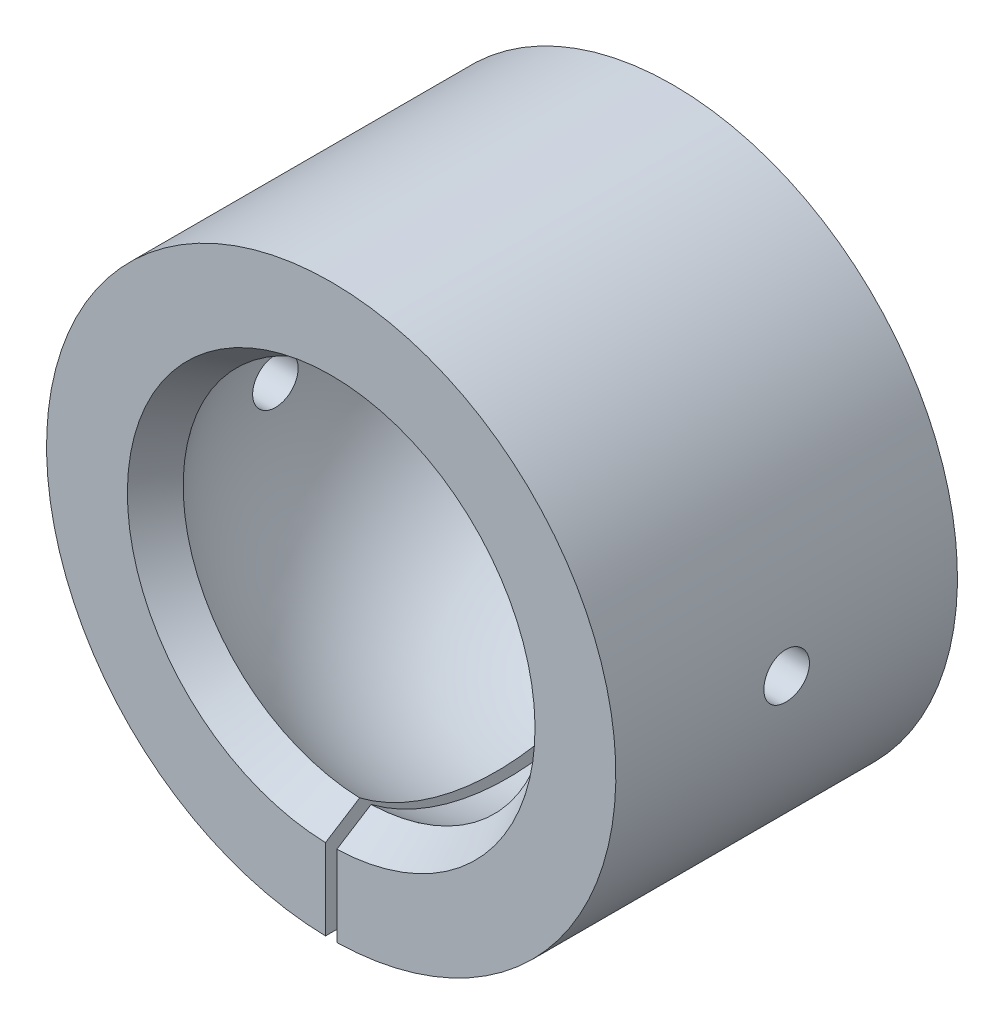
from build123d import *

# Parameters (mm, degrees)
SKETCH2_W               = 1
SKETCH2_H               = 35
CUT_EXTRUDE1_DEPTH      = 39.405728739
CUT_EXTRUDE2_DEPTH      = 39.405728739
CUT_EXTRUDE2_DEPTH_BACK = 39.405728739
SKETCH3_R               = 2


with BuildPart() as part:
    # Sketch1 → Revolve1 (revolve)
    with BuildSketch(Plane(origin=(0, 0, 0), x_dir=(1, 0, 0), z_dir=(0, 1, 0))):
        with BuildLine():
            Line((17.9, -15), (16, -12))
            ThreePointArc((16, -12), (19.895478191, 2.042044945), (13.228756555, 15))
            Line((13.228756555, 15), (25, 15))
            Line((25, 15), (25, -15))
            Line((25, -15), (17.9, -15))
        make_face()
    revolve(axis=Axis((0, 0, -23.629385965), (0, 0, 1)))

    # Sketch2 → Cut-Extrude1 (cut, through all)
    with BuildSketch(Plane(origin=(0, 0, 0), x_dir=(1, 0, 0), z_dir=(0, 1, 0))):
        Rectangle(SKETCH2_W, SKETCH2_H)
    extrude(amount=-CUT_EXTRUDE1_DEPTH, mode=Mode.SUBTRACT)

    # Sketch3 → Cut-Extrude2 (cut, two sides: drawn at the far end of the back side and taken through both)
    with BuildSketch(Plane(origin=(0, 0, 0), x_dir=(0, 0, -1), z_dir=(1, 0, 0)).offset(-CUT_EXTRUDE2_DEPTH_BACK)):
        Circle(SKETCH3_R)
    extrude(amount=CUT_EXTRUDE2_DEPTH + CUT_EXTRUDE2_DEPTH_BACK, mode=Mode.SUBTRACT)


solid = part.part
